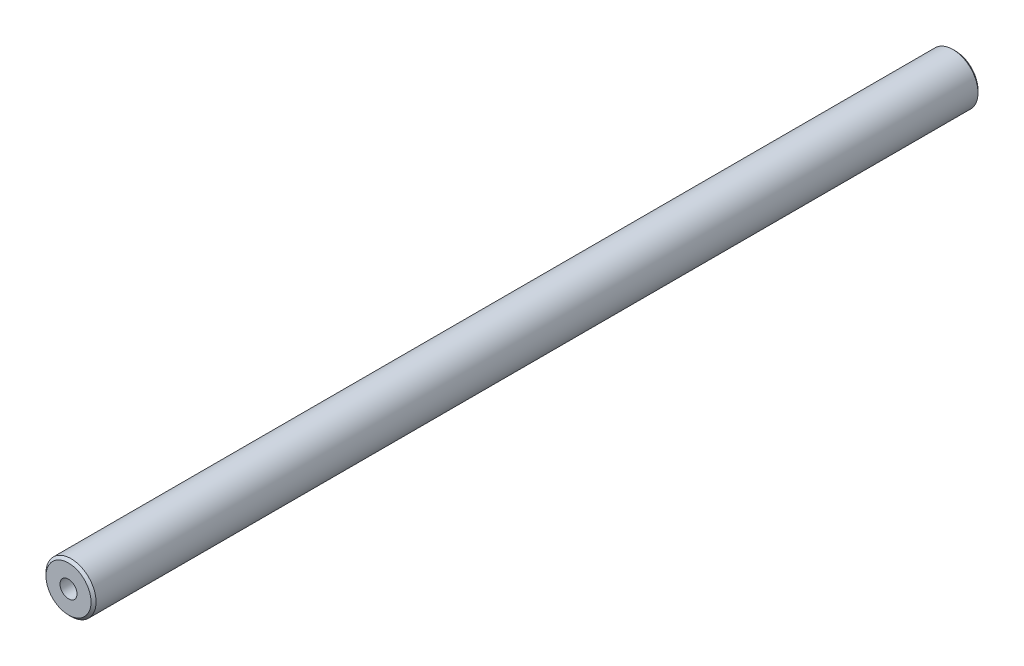
SolidWorks part; units mm, degrees
material "Q235A"
ref_plane "前视基准面" through (0, 0, 0) normal (0, 0, 1) x (1, 0, 0)
ref_plane "上视基准面" through (0, 0, 0) normal (0, 1, 0) x (1, 0, 0)
ref_plane "右视基准面" through (0, 0, 0) normal (1, 0, 0) x (0, 0, -1)
sketch "草图1" plane through (0, 0, 0) normal (0, 0, 1) x (1, 0, 0)
  circle A0 centre (0, 0) radius 10
  dimension "D1" = 20
extrude "凸台-拉伸1" add sketch "草图1" along normal mid plane 354
hole_wizard "M8 螺纹孔1" positions "草图2" profile "草图3" tap size "M8" standard "ISO"
sketch "草图2" plane through (0, 0, -177) normal (0, 0, -1) x (-1, 0, 0)
  point P0 (0, 0)
sketch "草图3" plane through (0, 0, -177) normal (1, 0, 0) x (0, 1, 0)
  line L0 (0, 0) -> (0, 21.7929)
  line L1 (0, 21.7929) -> (3.4, 19.75)
  line L2 (3.4, 19.75) -> (3.4, 0)
  line L5 (3.4, 0) -> (0, 0)
  line L10 (0, 21.7929) -> (-3.4, 19.75) construction
  line L11 (0, -6.35) -> (0, 107.95) construction
  dimension "螺纹孔钻头直径" = 6.8
  dimension "螺纹孔钻头深度" = 19.75
  dimension "导头角度" = 118
cosmetic thread "孔螺蚊线1"
hole_wizard "M8 螺纹孔2" positions "草图4" profile "草图5" tap size "M8" standard "ISO"
sketch "草图4" plane through (0, 0, 177) normal (0, 0, 1) x (1, 0, 0)
  point P0 (0, 0)
sketch "草图5" plane through (0, 0, 177) normal (1, 0, 0) x (0, -1, 0)
  line L0 (0, 0) -> (0, 21.7929)
  line L1 (0, 21.7929) -> (3.4, 19.75)
  line L2 (3.4, 19.75) -> (3.4, 0)
  line L5 (3.4, 0) -> (0, 0)
  line L10 (0, 21.7929) -> (-3.4, 19.75) construction
  line L11 (0, -6.35) -> (0, 107.95) construction
  dimension "螺纹孔钻头直径" = 6.8
  dimension "螺纹孔钻头深度" = 19.75
  dimension "导头角度" = 118
cosmetic thread "孔螺蚊线2"
chamfer "倒角1" distance 1 angle 45 2 edges at (10, 0, -177) (10, 0, 177)
